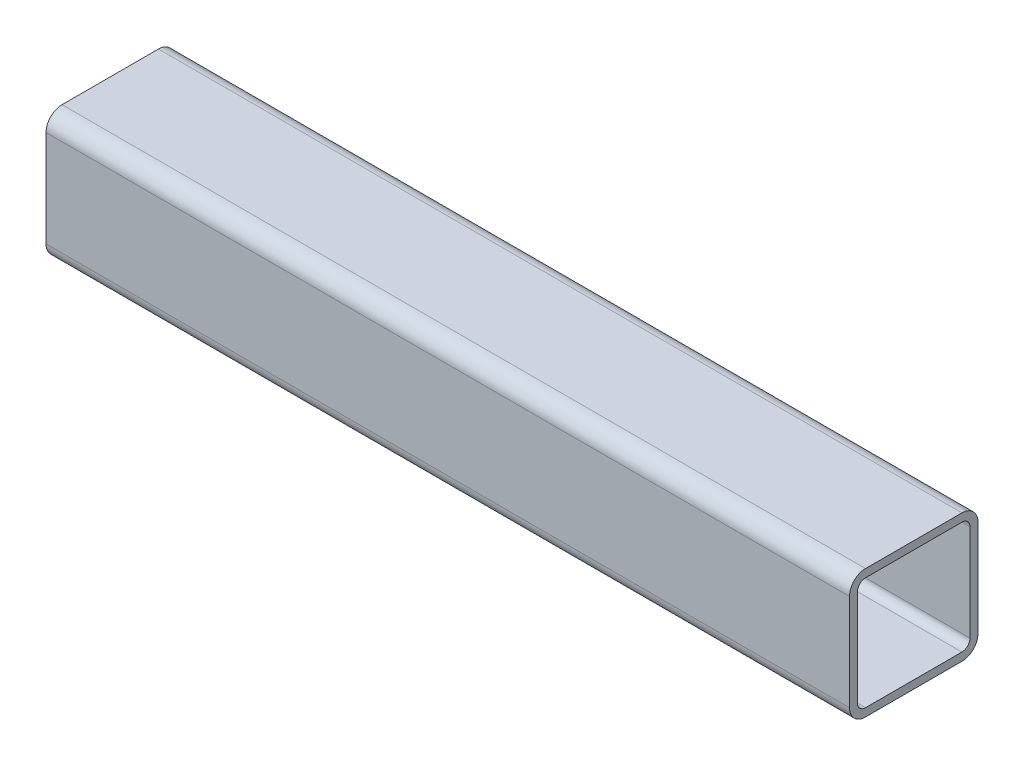
from build123d import *

# Parameters (mm, degrees)
SQUARE_TUBE_80_X_80_X_5_0_1_DEPTH = 500


with BuildPart() as part:
    # Sketch1 → Square Tube 80 X 80 X 5.0(1) (new body)
    with BuildSketch(Plane(origin=(-250, 0, 0), x_dir=(0, 0, -1), z_dir=(1, 0, 0))):
        with BuildLine():
            Line((-30, -40), (30, -40))
            ThreePointArc((30, -40), (37.071067812, -37.071067812), (40, -30))
            Line((40, -30), (40, 30))
            ThreePointArc((40, 30), (37.071067812, 37.071067812), (30, 40))
            Line((30, 40), (-30, 40))
            ThreePointArc((-30, 40), (-37.071067812, 37.071067812), (-40, 30))
            Line((-40, 30), (-40, -30))
            ThreePointArc((-40, -30), (-37.071067812, -37.071067812), (-30, -40))
        make_face()
        with BuildLine():
            Line((-30, -35), (30, -35))
            ThreePointArc((30, -35), (33.535533906, -33.535533906), (35, -30))
            Line((35, -30), (35, 30))
            ThreePointArc((35, 30), (33.535533906, 33.535533906), (30, 35))
            Line((30, 35), (-30, 35))
            ThreePointArc((-30, 35), (-33.535533906, 33.535533906), (-35, 30))
            Line((-35, 30), (-35, -30))
            ThreePointArc((-35, -30), (-33.535533906, -33.535533906), (-30, -35))
        make_face(mode=Mode.SUBTRACT)
    extrude(amount=SQUARE_TUBE_80_X_80_X_5_0_1_DEPTH)


solid = part.part
